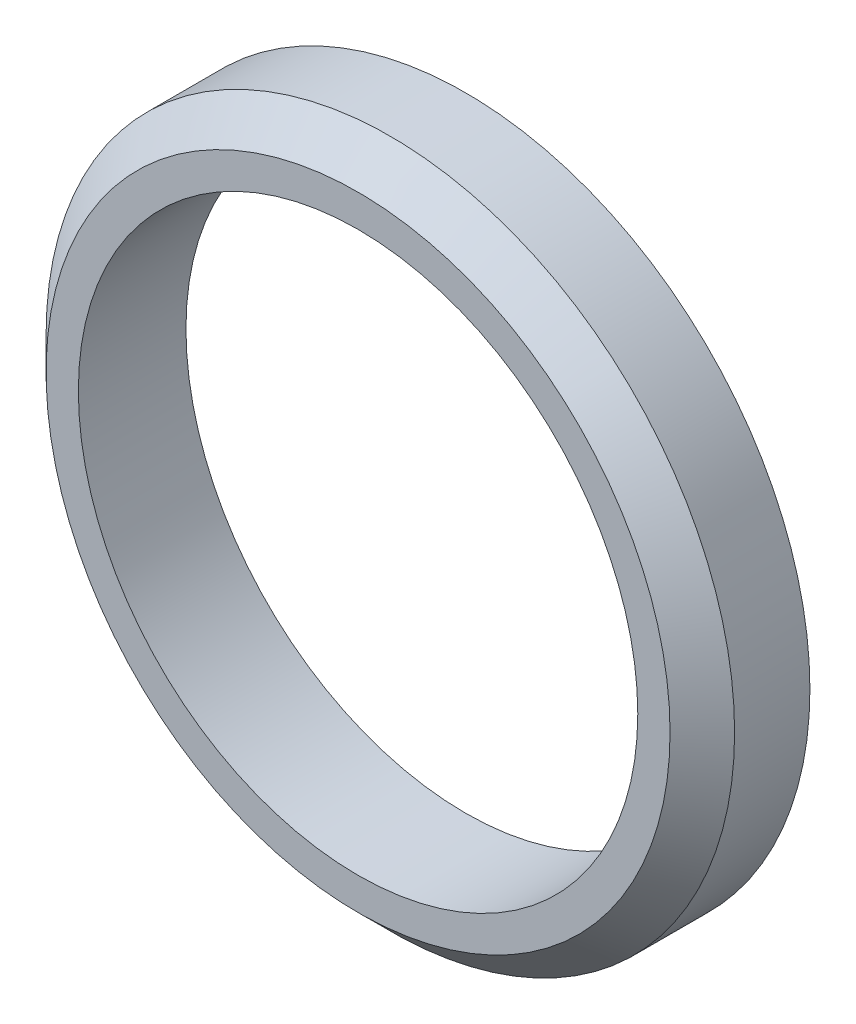
SolidWorks part; units mm, degrees
ref_plane "Front Plane" through (0, 0, 0) normal (0, 0, 1) x (1, 0, 0)
ref_plane "Top Plane" through (0, 0, 0) normal (0, 1, 0) x (1, 0, 0)
ref_plane "Right Plane" through (0, 0, 0) normal (1, 0, 0) x (0, 0, -1)
sketch "Sketch1" plane through (0, 0, 0) normal (0, 0, 1) x (1, 0, 0)
  circle A0 centre (0, 0) radius 16
  circle A1 centre (0, 0) radius 13
  dimension "D1" = 32
  dimension "D2" = 26
extrude "Boss-Extrude1" add sketch "Sketch1" along normal blind 5
chamfer "Chamfer1" distance 1.5 angle 45 1 edges at (16, 0, 5)
